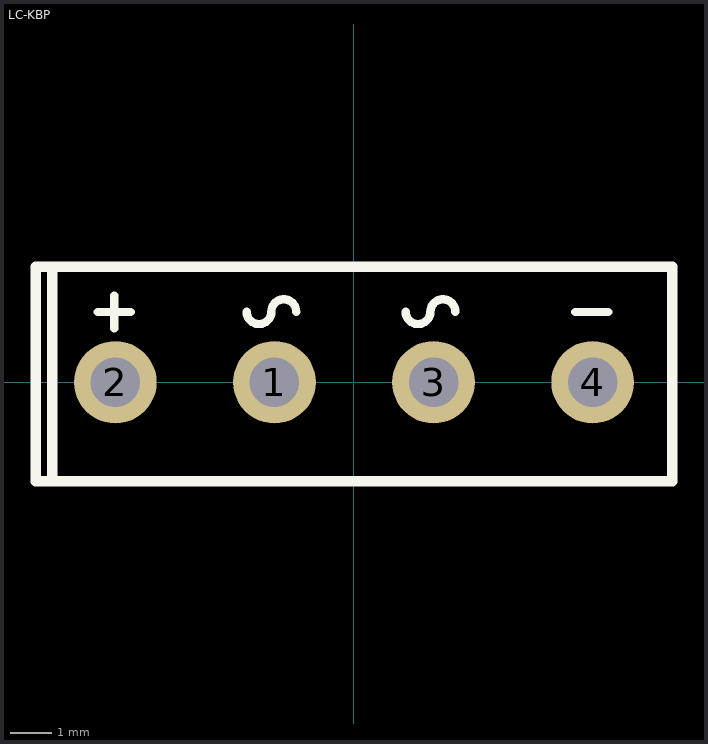
[diagram p0: the footprint, top view; thin cyan lines are the x and y axes]
# Altium footprint library MISC89340-8.PcbLib: 1 footprints
Each footprint in its own frame and in the unit in brackets; x right, y up, seen from the top. Pads: shape width x height; smd on the part's side, far side on the other; paste and mask are expansions set on the pad; w line width, h text height; cw(c..) or ccw(c..) is an arc to the next point about the centre after c.

## LC-KBP [mm]
pads (4):
  round 2 hole 1.2: 1(-1.925,0) 2(-5.775,0) 3(1.925,0) 4(5.775,0)
Top Overlay:
  lines w0.203: -6.2,1.7 -5.4,1.7 ; -5.8,1.3 -5.8,2.1 ; -2.6,1.708 ccw(c-2.3,1.708) -2,1.708 cw(c-1.7,1.708) -1.4,1.708 ; 1.25,1.708 ccw(c1.55,1.708) 1.85,1.708 cw(c2.15,1.708) 2.45,1.708 ; 5.35,1.7 6.15,1.7
  lines w0.254: -7.3,-2.4 -7.3,2.8 ; -7.7,-2.4 7.7,-2.4 7.7,2.8 -7.7,2.8 -7.7,-2.4